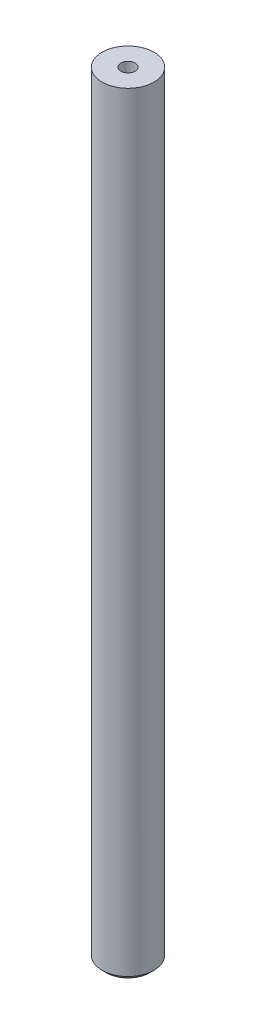
SolidWorks part; units mm, degrees
ref_plane "Front Plane" through (0, 0, 0) normal (0, 0, 1) x (1, 0, 0)
ref_plane "Top Plane" through (0, 0, 0) normal (0, 1, 0) x (1, 0, 0)
ref_plane "Right Plane" through (0, 0, 0) normal (1, 0, 0) x (0, 0, -1)
sketch "Sketch1" plane through (0, 0, 0) normal (0, 1, 0) x (1, 0, 0)
  circle A0 centre (0, 0) radius 6
  dimension "D1" = 12
extrude "Boss-Extrude1" add sketch "Sketch1" along normal blind 179
hole_wizard "M4 Tapped Hole1" positions "Sketch2" profile "Sketch3" tap size "M4" standard "GB"
sketch "Sketch2" plane through (0, 179, 0) normal (0, 1, 0) x (1, 0, 0)
  point P0 (0, 0)
  point P3 (-123.2576, 97.2449)
  point P6 (-195.1073, 6.1756)
  point P9 (-71.8497, -91.0693)
cosmetic thread "Cosmetic Thread1" parameters "D1"=179, "D2"=4
sketch "Sketch3" plane through (0, 179, 0) normal (1, 0, 0) x (0, 0, 1)
  line L0 (0, 0) -> (0, 30.9914)
  line L1 (0, 30.9914) -> (1.65, 30)
  line L2 (1.65, 30) -> (1.65, 0)
  line L5 (1.65, 0) -> (0, 0)
  line L10 (0, 30.9914) -> (-1.65, 30) construction
  line L11 (0, -6.35) -> (0, 107.95) construction
  dimension "螺纹孔钻头直径" = 3.3
  dimension "螺纹孔钻头深度" = 30
  dimension "导头角度" = 118
chamfer "Chamfer1" distance 1 angle 45 1 edges at (0, 0, 6)
equation "\"1\"= \"代号代号\""
equation "\"2\"= \"名称代号\""
